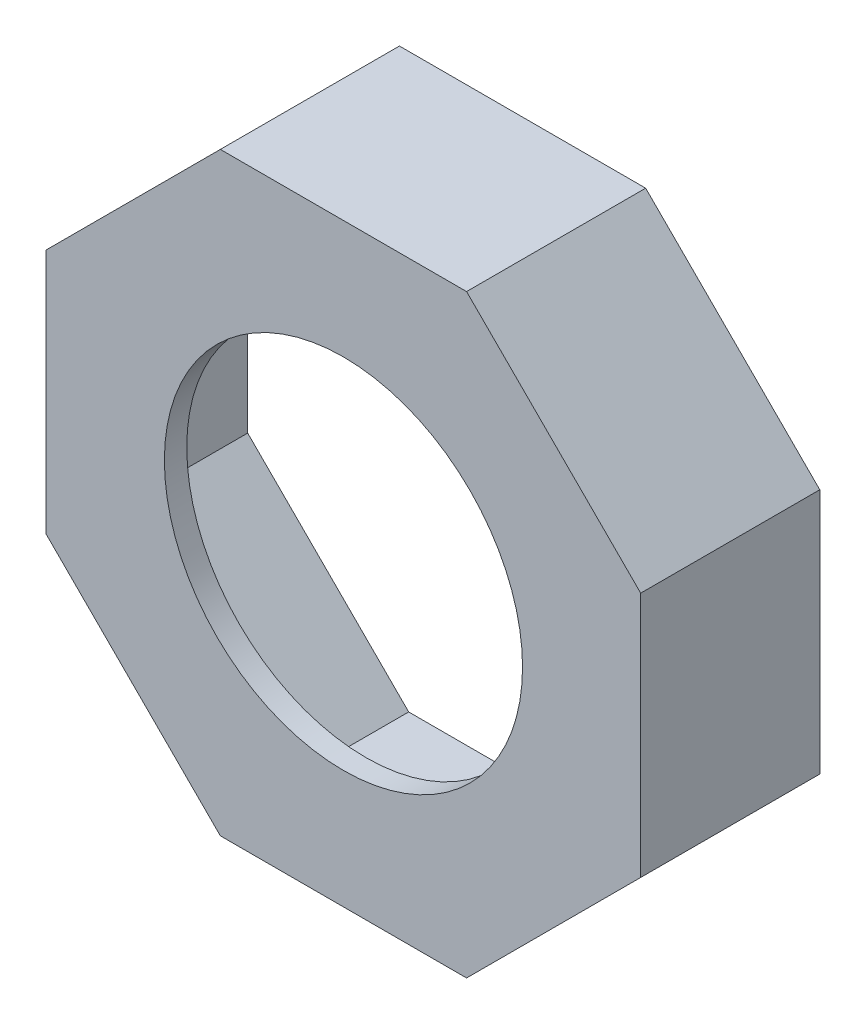
from build123d import *

# Parameters (mm, degrees)
BOSS_EXTRUDE1_DEPTH = 80
SHELL1_T            = -10
SKETCH2_R           = 80
CUT_EXTRUDE1_DEPTH  = 80


with BuildPart() as part:
    # Sketch1 → Boss-Extrude1 (new body)
    with BuildSketch(Plane.XY):
        Polygon((-467.102450828, -35), (-544.884196758, 42.781745931), (-654.884196758, 42.781745931), (-732.665942689, -35), (-732.665942689, -145), (-654.884196758, -222.781745931), (-544.884196758, -222.781745931), (-467.102450828, -145), align=None)
    extrude(amount=BOSS_EXTRUDE1_DEPTH)

    # Shell1
    shell1_openings = [part.faces().sort_by_distance(p)[0] for p in [
        (-599.884196758, -90, 0),
    ]]
    offset(amount=SHELL1_T, openings=shell1_openings, kind=Kind.INTERSECTION)

    # Sketch2 → Cut-Extrude1 (cut)
    with BuildSketch(Plane.XY.offset(80)):
        with Locations((-599.884196758, -90)):
            Circle(SKETCH2_R)
    extrude(amount=-CUT_EXTRUDE1_DEPTH, mode=Mode.SUBTRACT)


solid = part.part
